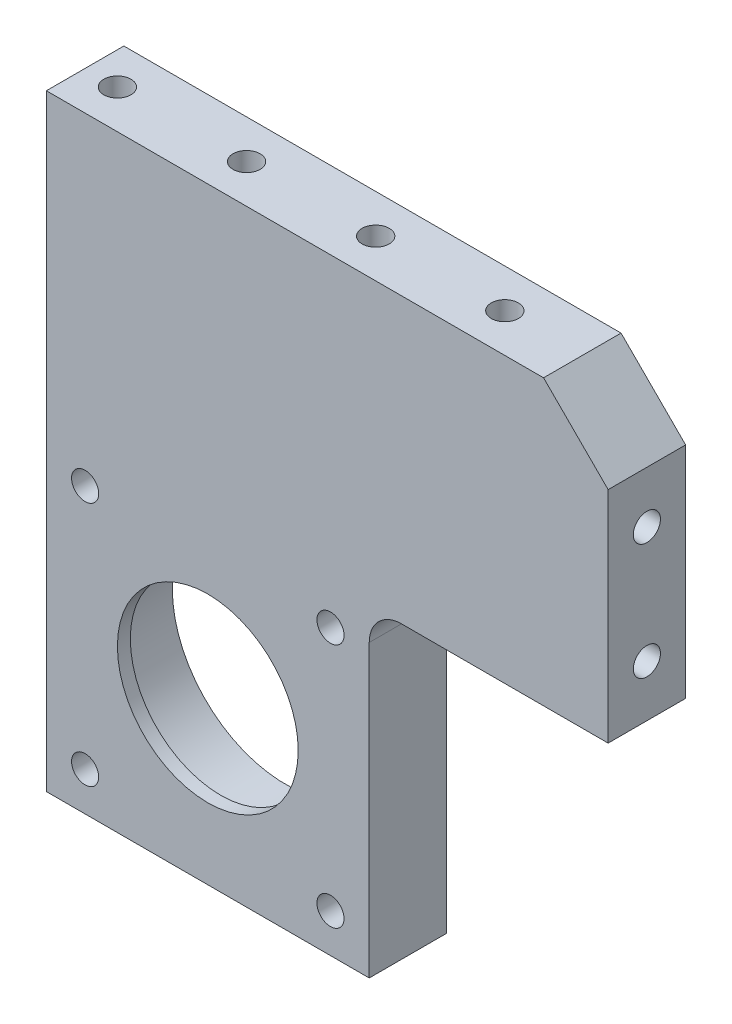
from build123d import *

# Parameters (mm, degrees)
SKETCH_1_W             = 105
SKETCH_1_H             = 95
EXTRUDE_1_DEPTH        = 6
SKETCH_10_R            = 17.5
CUT_EXTRUDE_1_DEPTH    = 10
SKETCH_12_R            = 14
CUT_EXTRUDE_2_DEPTH    = 72.50174823
SKETCH_13_W            = 55
SKETCH_13_H            = 50
CUT_EXTRUDE_3_DEPTH    = 72.808773837
FILLET_1_R             = 5
HOLE_WIZARD_M5_2_D     = 4.2
MOVE_FACE_1_BY         = 1
MOVE_FACE_2_BY         = 18
CHAMFER_2_SIZE         = 10
HOLE_WIZARD_M5_3_D     = 4.2
HOLE_WIZARD_M5_3_DEPTH = 12.4
HOLE_WIZARD_M5_3_TIP   = 1.2618073
HOLE_WIZARD_M5_4_D     = 4.2
HOLE_WIZARD_M5_4_DEPTH = 12.4
HOLE_WIZARD_M5_4_TIP   = 1.2618073


with BuildPart() as part:
    # 草图1 → 凸台-拉伸1 (new, symmetric)
    with BuildSketch(Plane.XY):
        Rectangle(SKETCH_1_W, SKETCH_1_H)
    extrude(amount=EXTRUDE_1_DEPTH, both=True)

    # 草图10 → 切除-拉伸1 (cut)
    with BuildSketch(Plane.XY.offset(-6)):
        with Locations((-27.5, -22.5)):
            Circle(SKETCH_10_R)
    extrude(amount=CUT_EXTRUDE_1_DEPTH, mode=Mode.SUBTRACT)

    # 草图12 → 切除-拉伸2 (cut, through all)
    with BuildSketch(Plane(origin=(0, 0, 4), x_dir=(-1, 0, 0), z_dir=(0, 0, -1))):
        with Locations((27.5, -22.5)):
            Circle(SKETCH_12_R)
    extrude(amount=-CUT_EXTRUDE_2_DEPTH, mode=Mode.SUBTRACT)

    # 草图13 → 切除-拉伸3 (cut, through all)
    with BuildSketch(Plane.XY.offset(6)):
        with Locations((25, -22.5)):
            Rectangle(SKETCH_13_W, SKETCH_13_H)
    extrude(amount=-CUT_EXTRUDE_3_DEPTH, mode=Mode.SUBTRACT)

    # 圆角1
    fillet_1_edges = [part.edges().sort_by_distance(p)[0] for p in [
        (-2.5, 2.5, 0),
    ]]
    fillet(fillet_1_edges, radius=FILLET_1_R)

    # M5 螺纹孔2 (through all)
    with Locations(Plane(origin=(0, 0, -6), x_dir=(-1, 0, 0), z_dir=(0, 0, -1))):
        with Locations((8.5, -3.5), (8.5, -41.5), (46.5, -41.5), (46.5, -3.5)):
            Hole(HOLE_WIZARD_M5_2_D / 2)

    # Move Face 1: a face moved inward by 1.0
    extrude(part.faces().sort_by_distance((0, 47.5, 0))[0], amount=MOVE_FACE_1_BY, dir=(0, -1, 0), mode=Mode.SUBTRACT)

    # Move Face 2: a face moved inward by 18.0
    extrude(part.faces().sort_by_distance((52.5, 24.5, 0))[0], amount=MOVE_FACE_2_BY, dir=(-1, 0, 0), mode=Mode.SUBTRACT)

    # 倒角2
    chamfer_2_edges = [part.edges().sort_by_distance(p)[0] for p in [
        (34.5, 46.5, 0),
    ]]
    chamfer(chamfer_2_edges, length=CHAMFER_2_SIZE)

    # M5 螺纹孔3
    with Locations(Plane(origin=(0, 46.5, 0), x_dir=(1, 0, 0), z_dir=(0, 1, 0))):
        with Locations((12.5, 0), (-7.5, 0), (-27.5, 0), (-47.5, 0)):
            Hole(HOLE_WIZARD_M5_3_D / 2, depth=HOLE_WIZARD_M5_3_DEPTH)
            with Locations((0, 0, -(HOLE_WIZARD_M5_3_DEPTH + HOLE_WIZARD_M5_3_TIP / 2))):  # 118° drill point
                Cone(0, HOLE_WIZARD_M5_3_D / 2, HOLE_WIZARD_M5_3_TIP, mode=Mode.SUBTRACT)

    # M5 螺纹孔4
    with Locations(Plane(origin=(34.5, 0, 0), x_dir=(0, 0, -1), z_dir=(1, 0, 0))):
        with Locations((0, 28.5), (0, 10.5)):
            Hole(HOLE_WIZARD_M5_4_D / 2, depth=HOLE_WIZARD_M5_4_DEPTH)
            with Locations((0, 0, -(HOLE_WIZARD_M5_4_DEPTH + HOLE_WIZARD_M5_4_TIP / 2))):  # 118° drill point
                Cone(0, HOLE_WIZARD_M5_4_D / 2, HOLE_WIZARD_M5_4_TIP, mode=Mode.SUBTRACT)


solid = part.part
